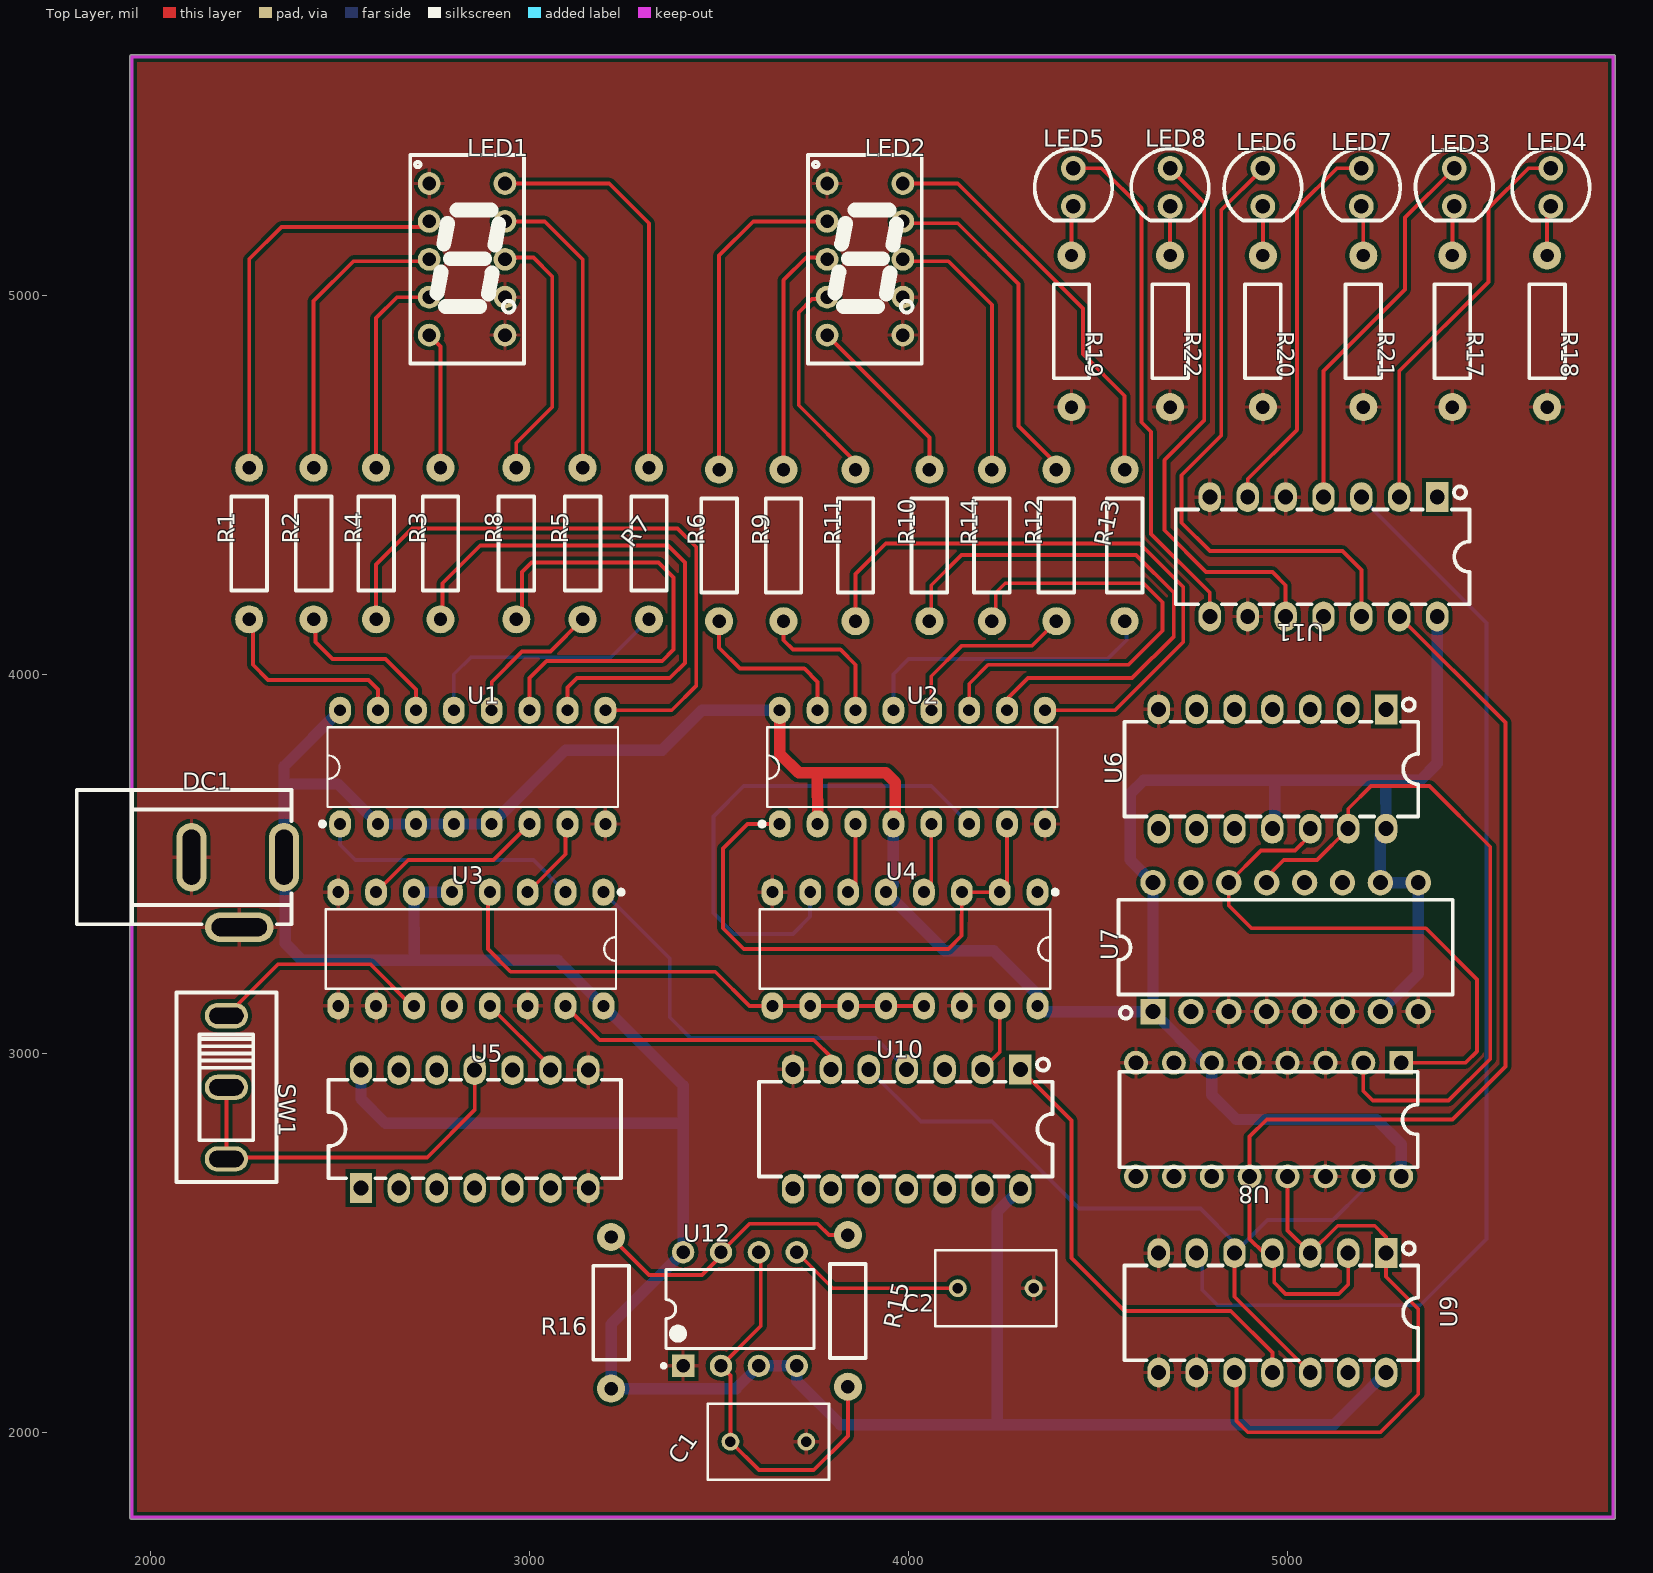
[diagram p0: Top Layer view]
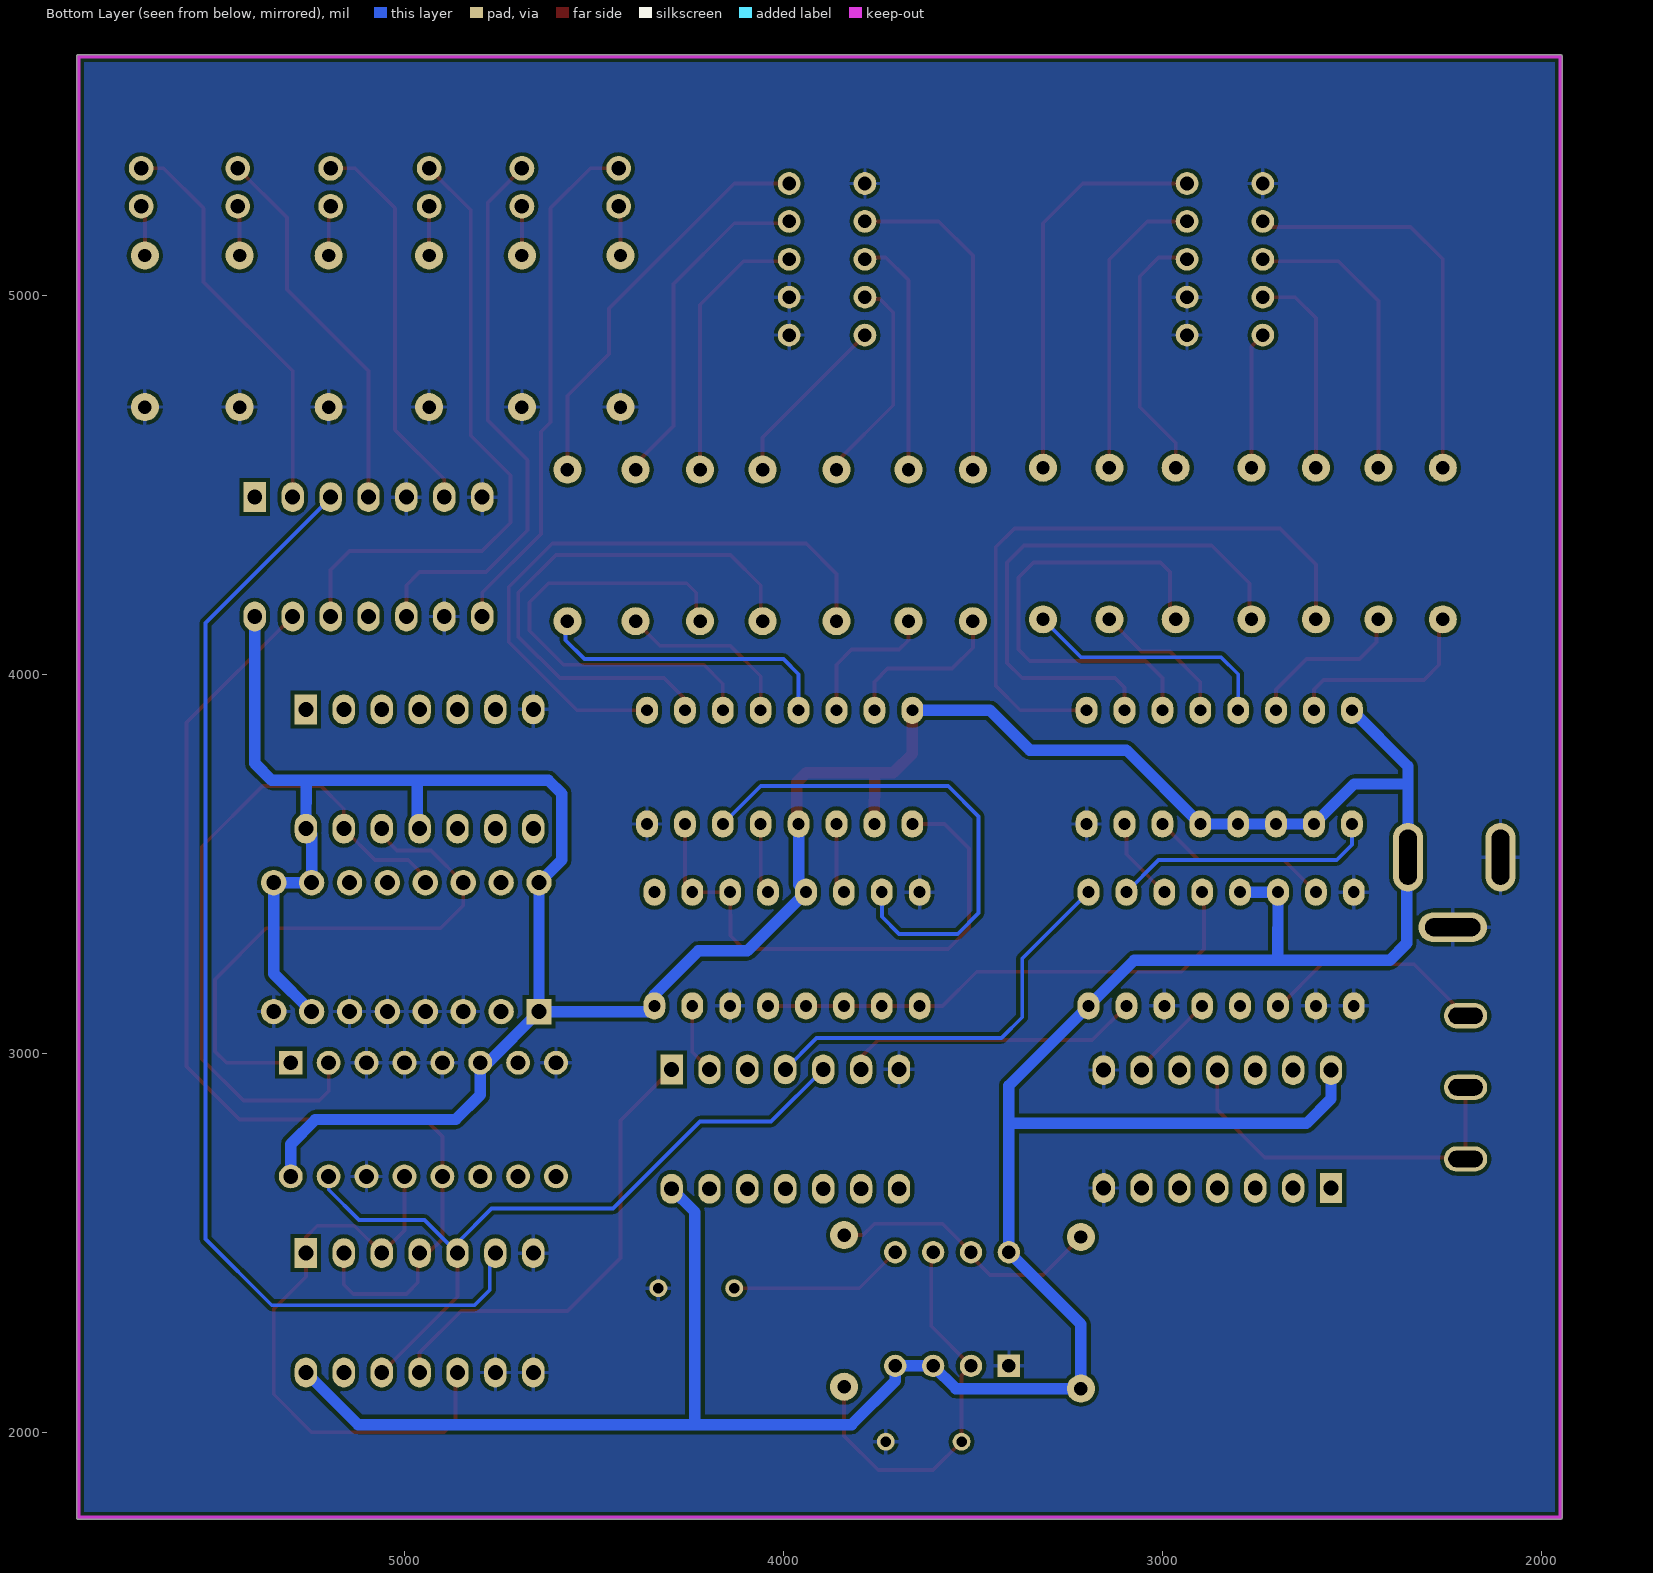
[diagram p1: Bottom Layer view, seen from below]
# Altium PCB MISC80800.pcbdoc
Units mil, origin at the board's own origin, x right, y up, seen from the top; angles counter-clockwise.
Board outline 3920.03 x 3865.03 mil, 2 copper layers (Top Layer, Bottom Layer); 46 components, 74 nets, 260 pads, 0 vias.

## Layer stack, top to bottom (the 12.6 mil dielectric is the usual default, probably not edited)
Top Solder: solder mask 0.4, Solder Resist, Dk 3.5
Top Layer: signal copper 1.4
Dielectric1: dielectric 12.6, FR-4, Dk 4.8
Bottom Layer: signal copper 1.4
Bottom Solder: solder mask 0.4, Solder Resist, Dk 3.5

## Board outline
1944.98,1775 ccw(c1950,1775) 1950,1769.98 5860,1769.98 ccw(c5860,1775) 5865.02,1775 5865.02,5630 ccw(c5860,5630) 5860,5635.02 1950,5635.02 ccw(c1950,5630) 1944.98,5630

## Design rules (kind name [scope] priority, off if disabled: settings)
Clearance [All] p1: gap=10
HoleSize [All] p1: absolutevalues=TRUE maxlimit=6666 minlimit=1 maxpercent=80.000 minpercent=20.000
MinimumSolderMaskSliver [All] p1: minsoldermaskwidth=0
PolygonConnect [All] p1: connectstyle=Relief reliefconductorwidth=10 reliefentries=4 polygonreliefangle="90 Angle" airgapwidth=10
RoutingVias [All] p1: holewidth=28 width=50 viastyle="Through Hole" minholewidth=28 minwidth=50 maxholewidth=28 maxwidth=50
SilkToSilkClearance [All] p1: silktosilkclearance=0
SilkToSolderMaskClearance [IsPad] p1: minsilkscreentomaskgap=0 clearancetoexposedcopper=TRUE
SolderMaskExpansion [All] p1: expansion=4
Width [All] p1: maxlimit=50 minlimit=10 preferedwidth=10
26 further rules are at their usual default settings.

## Components (designator, comment, footprint, x,y, rotation, side; value= is the part's Value field where it differs from the comment)
C1 "10U" RAD-0.2 3630,1975 r180 top
C2 "10N" RAD-0.2 4230,2380 r180 top
DC1 "DC005-2.0MM" DC-IN-TH_DC005 2230,3425 r0 top
LED1 "FJ3161AH" LED-SEG-TH_10P-L14.0-W7.5-P2.54-S5.08-TL 2835,5095 r0 top
LED2 "FJ3161AH" LED-SEG-TH_10P-L14.0-W7.5-P2.54-S5.08-TL 3885,5095 r0 top
LED3 "LED-TH-5mm_R" LED-TH_BD5.0_RED 5440,5285 r0 top
LED4 "LED-TH-5mm_R" LED-TH_BD5.0_RED 5695,5284.99 r0 top
LED5 "LED-TH-5mm_R" LED-TH_BD5.0_RED 4435,5284.99 r0 top
LED6 "LED-TH-5mm_R" LED-TH_BD5.0_RED 4935,5284.99 r0 top
LED7 "LED-TH-5mm_R" LED-TH_BD5.0_RED 5195,5284.99 r0 top
LED8 "LED-TH-5mm_R" LED-TH_BD5.0_RED 4690,5285 r0 top
R1 "330" R_AXIAL-0.4 2260,4345 r90 top
R2 "330" R_AXIAL-0.4 2430,4345 r90 top
R3 "330" R_AXIAL-0.4 2765,4345 r90 top
R4 "330" R_AXIAL-0.4 2595,4345 r90 top
R5 "330" R_AXIAL-0.4 3140,4345 r90 top
R6 "330" R_AXIAL-0.4 3500,4340 r90 top
R7 "330" R_AXIAL-0.4 3315,4345 r90 top
R8 "330" R_AXIAL-0.4 2965,4345 r90 top
R9 "330" R_AXIAL-0.4 3670,4340 r90 top
R10 "330" R_AXIAL-0.4 4055,4340 r90 top
R11 "330" R_AXIAL-0.4 3860,4340 r90 top
R12 "330" R_AXIAL-0.4 4390,4340 r90 top
R13 "330" R_AXIAL-0.4 4570,4340 r90 top
R14 "330" R_AXIAL-0.4 4220,4340 r90 top
R15 "50K" R_AXIAL-0.4 3840,2320 r270 top
R16 "50K" R_AXIAL-0.4 3215,2315 r90 top
R17 "200" R_AXIAL-0.4 5435,4905 r270 top
R18 "200" R_AXIAL-0.4 5685,4905 r270 top
R19 "200" R_AXIAL-0.4 4430,4905 r270 top
R20 "200" R_AXIAL-0.4 4935,4905 r270 top
R21 "200" R_AXIAL-0.4 5200,4905 r270 top
R22 "200" R_AXIAL-0.4 4690,4905 r270 top
SW1 "SS12D10G4 071" SW-TH_SHOU-HAN_SS12D10G4 2200,2910 r270 top
U1 "XD74LS48" DIP-16_L19.3-W6.4-P2.54-LS7.6-BL 2850,3755 r0 top
U2 "XD74LS48" DIP-16_L19.3-W6.4-P2.54-LS7.6-BL 4010,3755 r0 top
U3 "XD74LS192" DIP-16_L19.3-W6.4-P2.54-LS7.6-BL 2845,3275 r180 top
U4 "XD74LS192" DIP-16_L19.3-W6.4-P2.54-LS7.6-BL 3990.56,3275 r180 top
U5 "SN74LS32N" PDIP-14_L19.6-W6.5-P2.54-LS7.9-BL 2855,2800 r0 top
U6 "SN74LS00N" PDIP-14_L19.7-W6.6-P2.54-LS8.3-BL 4960,3750 r180 top
U7 "SN74LS160N(LX)" DIP-16_L22.4-W6.4-P2.54-LS8.64-BL 4995,3280 r0 top
U8 "XD74LS138" DIP-16_L19.8-W6.5-P2.54-LS7.6-BL 4950,2825 r180 top
U9 "SN74LS00N" PDIP-14_L19.7-W6.6-P2.54-LS8.3-BL 4960,2315 r180 top
U10 "SN74LS04N" PDIP-14_L19.7-W6.6-P2.54-LS8.3-BL 3995,2800 r180 top
U11 "SN74LS04N" PDIP-14_L19.7-W6.6-P2.54-LS8.3-BL 5095,4310 r180 top
U12 "100kHz" DIP-8_L9.8-W6.6-P2.54-LS7.6-BL 3555,2325 r0 top

## Footprints (in the part's own frame and the unit in brackets; to place one, negate y for a bottom-side part, rotate by r counter-clockwise, add the part's x,y. Pads: shape width x height; smd on the part's side, far side on the other; paste and mask are expansions set on the pad)
DC-IN-TH_DC005 [mm]
  oval 2x4.6 hole 1.2 slot 3.7 at 90 deg paste+0 mask+0.051: 1(3.1,2.35) 2(-3.1,2.35)
  oval 4.6x2 hole 1.2 slot 3.7 at 0 deg paste+0 mask+0.051: 3(0.1,-2.35)
  silkscreen extent -10.8,-2.15 3.6,6.85
DIP-8_L9.8-W6.6-P2.54-LS7.6-BL [mm]
  rect 1.5x1.5 hole 0.9 paste+0 mask+0.051: 1(-3.81,-3.81)
  round 1.5 hole 0.9 paste+0 mask+0.051: 2(-1.27,-3.81) 3(1.27,-3.81) 4(3.81,-3.81) 5(3.81,3.81) 6(1.27,3.81) 7(-1.27,3.81) 8(-3.81,3.81)
  silkscreen extent -5.23,-3.93 4.96,2.65
DIP-16_L19.3-W6.4-P2.54-LS7.6-BL [mm]
  oval 1.46x1.825 hole 0.8 paste+0 mask+0.051: 1(-8.89,-3.81) 2(-6.35,-3.81) 3(-3.81,-3.81) 4(-1.27,-3.81) 5(1.27,-3.81) 6(3.81,-3.81) 7(6.35,-3.81) 8(8.89,-3.81) 9(8.89,3.81) 10(6.35,3.81) 11(3.81,3.81) 12(1.27,3.81) 13(-1.27,3.81) 14(-3.81,3.81) 15(-6.35,3.81) 16(-8.89,3.81)
  silkscreen extent -10.22,-3.96 9.73,2.67
DIP-16_L19.8-W6.5-P2.54-LS7.6-BL [mm]
  rect 1.6x1.6 hole 1 paste+0 mask+0.051: 1(-8.89,-3.81)
  round 1.6 hole 1 paste+0 mask+0.051: 2(-6.35,-3.81) 3(-3.81,-3.81) 4(-1.27,-3.81) 5(1.27,-3.81) 6(3.81,-3.81) 7(6.35,-3.81) 8(8.89,-3.81) 9(8.89,3.81) 10(6.35,3.81) 11(3.81,3.81) 12(1.27,3.81) 13(-1.27,3.81) 14(-3.81,3.81) 15(-6.35,3.81) 16(-8.89,3.81)
  silkscreen extent -10,-3.2 10,3.2
DIP-16_L22.4-W6.4-P2.54-LS8.64-BL [mm]
  rect 1.7x1.7 hole 1 paste+0 mask+0.051: 1(-8.89,-4.32)
  round 1.7 hole 1 paste+0 mask+0.051: 2(-6.35,-4.32) 3(-3.81,-4.32) 4(-1.27,-4.32) 5(1.27,-4.32) 6(3.81,-4.32) 7(6.35,-4.32) 8(8.89,-4.32) 9(8.89,4.32) 10(6.35,4.32) 11(3.81,4.32) 12(1.27,4.32) 13(-1.27,4.32) 14(-3.81,4.32) 15(-6.35,4.32) 16(-8.89,4.32)
  silkscreen extent -11.21,-4.79 11.2,3.18
LED-SEG-TH_10P-L14.0-W7.5-P2.54-S5.08-TL [mil]
  round 60 hole 36 paste+0 mask+2: 1(-100,200) 2(-100,100) 3(-100,0) 4(-100,-100) 5(-100,-200) 6(100,-200) 7(100,-100) 8(100,0) 9(100,100) 10(100,200)
  silkscreen extent -150,-275 150,275
LED-TH_BD5.0_RED [mil]
  round 65 hole 38 paste+0 mask+2: 1(0,50) 2(0,-50)
  silkscreen extent -102,-88 102,102
PDIP-14_L19.6-W6.5-P2.54-LS7.9-BL [mm]
  rect 1.5x2 hole 1 paste+0 mask+0.051: 1(-7.62,-3.95)
  oval 1.5x2 hole 1 paste+0 mask+0.051: 2(-5.08,-3.95) 3(-2.54,-3.95) 4(0,-3.95) 5(2.54,-3.95) 6(5.08,-3.95) 7(7.62,-3.95) 8(7.62,3.95) 9(5.08,3.95) 10(2.54,3.95) 11(0,3.95) 12(-2.54,3.95) 13(-5.08,3.95) 14(-7.62,3.95)
  silkscreen extent -9.8,-3.3 9.8,3.3
PDIP-14_L19.7-W6.6-P2.54-LS8.3-BL [mm]
  rect 1.5x2 hole 1 paste+0 mask+0.051: 1(-7.62,-4)
  oval 1.5x2 hole 1 paste+0 mask+0.051: 2(-5.08,-4) 3(-2.54,-4) 4(0,-4) 5(2.54,-4) 6(5.08,-4) 7(7.62,-4) 8(7.62,4) 9(5.08,4) 10(2.54,4) 11(0,4) 12(-2.54,4) 13(-5.08,4) 14(-7.62,4)
  silkscreen extent -9.78,-4.72 9.91,3.18
R_AXIAL-0.4 [mil]
  round 74 hole 35.4 paste+0 mask+2: 1(-200,0) 2(200,0)
  silkscreen extent -124,-47 124,47
RAD-0.2 [mm]
  round 1.2 hole 0.7 paste+0 mask+0.05: 1(2.54,0) 2(-2.54,0)
  silkscreen extent -4.06,-2.54 4.06,2.54
SW-TH_SHOU-HAN_SS12D10G4 [mm]
  oval 1.7x2.9 hole 1.1 slot 2.3 at 90 deg paste+0 mask+0.05: 1(-4.8,0) 2(0,0) 3(4.8,0)
  silkscreen extent -6.35,-3.35 6.35,3.35

## Nets (pads, with @x,y where several pads share a name; then routed paths per layer and width w, separated by ;. In a path a pad name is that pad's centre, name@x,y a point inside that pad or via, vN(x,y) a via of type N, cw(c..) or ccw(c..) an arc to the next point about the centre after c; other vN are vias at no path point)
GND: C1.2 C2.2 DC1.2 DC1.3 LED1.1 LED1.6 LED1.7 LED2.1 LED2.6 LED2.7 R17.2 R18.2 R19.2 R20.2 R21.2 R22.2 U1.8 U2.8 U3.8 U3.9 U3.10 U3.14 U4.8 U4.14 U5.7 U5.8 U6.7 U7.3 U7.4 U7.5 U7.6 U7.8 U8.3 U8.4 U8.5 U8.8 U8.14 U9.7 U9.8 U9.9 U10.7 U11.5 U11.7 U11.9 U12.1
LED1_2: LED1.2 R1.2 | length 1066.4
  Top Layer w10: R1.2 2260,5095 2345,5180 2720,5180 LED1.2
LED1_3: LED1.3 R2.2 | length 790.6
  Top Layer w10: R2.2 2430,4985 2535,5090 2730,5090 LED1.3
LED1_4: LED1.4 R4.2 | length 557.8
  Top Layer w10: R4.2 2595,4940 2650,4995 LED1.4
LED1_5: LED1.5 R3.2 | length 362.4
  Top Layer w10: LED1.5 2765,4865 R3.2
LED1_8: LED1.8 R8.2 | length 692.1
  Top Layer w10: LED1.8 2940,5100 3010,5100 3060,5050 3060,4705 2965,4610 R8.2
LED1_9: LED1.9 R5.2 | length 796.4
  Top Layer w10: LED1.9 3040,5195 3140,5095 R5.2
LED1_10: LED1.10 R7.2 | length 1068.5
  Top Layer w10: LED1.10 3210,5295 3315,5190 R7.2
LED2_2: LED2.2 R6.2 | length 887.3
  Top Layer w10: R6.2 3500,5105 3590,5195 LED2.2
LED2_3: LED2.3 R9.2 | length 641.9
  Top Layer w10: R9.2 3670,5040 3730,5100 3780,5100 LED2.3
LED2_4: LED2.4 R11.2 | length 568.7
  Top Layer w10: LED2.4 3780,4990 3745,4990 3710,4955 3710,4710 3860,4560 R11.2
LED2_5: LED2.5 R10.2 | length 466.8
  Top Layer w10: LED2.5 4055,4625 R10.2
LED2_8: LED2.8 R14.2 | length 719.7
  Top Layer w10: LED2.8 3990,5090 4105,5090 4220,4975 R14.2
LED2_9: LED2.9 R12.2 | length 904.8
  Top Layer w10: LED2.9 3990,5190 4130,5190 4290,5030 4290,4655 4390,4555 R12.2
LED2_10: LED2.10 R13.2 | length 1082.3
  Top Layer w10: LED2.10 4130,5295 4460,4965 4460,4845 4570,4735 R13.2
LED3_2: LED3.2 R17.1 | length 132.1
  Top Layer w10: R17.1 5435,5230 LED3.2
LED5_2: LED5.2 R19.1 | length 132.1
  Top Layer w10: R19.1 4430,5229.99 LED5.2
LED7_2: LED7.2 R21.1 | length 132.1
  Top Layer w10: LED7.2 5200,5229.99 R21.1
R1_1: R1.1 U1.15 | length 536.1
  Top Layer w10: R1.1 2270,4135 2270,4025 2310,3985 2575,3985 2600,3960 U1.15
R2_1: R2.1 U1.14 | length 433.8
  Top Layer w10: R2.1 2435,4140 2435,4085 2480,4040 2620,4040 2700,3960 U1.14
R3_1: R3.1 U1.10 | length 1459.1
  Top Layer w10: R3.1 2770,4150 2770,4240 2870,4340 3365,4340 3410,4295 3410,4030 3370,3990 3125,3990 3100,3965 U1.10
R4_1: R4.1 U1.9 | length 1682
  Top Layer w10: R4.1 2595,4290 2690,4385 3390,4385 3440,4335 3440,3970 3375,3905 U1.9
R5_1: R5.1 U1.12 | length 383.3
  Top Layer w10: U1.12 2900,3980 2980,4060 3055,4060 R5.1
R6_1: R6.1 U2.15 | length 442.3
  Top Layer w10: R6.1 3500,4070 3555,4015 3725,4015 3760,3980 U2.15
R7_1: R7.1 U1.13 | length 670.1
  Bottom Layer w10: U1.13 2800,4000 2845,4045 3215,4045 R7.1
R8_1: R8.1 U1.11 | length 1244.2
  Top Layer w10: R8.1 2980,4160 2980,4270 3005,4295 3340,4295 3380,4255 3380,4065 3350,4035 3045,4035 3000,3990 U1.11
R9_1: R9.1 U2.14 | length 386.9
  Top Layer w10: R9.1 3670,4090 3695,4065 3820,4065 3860,4025 U2.14
R10_1: R10.1 U2.10 | length 1465
  Top Layer w10: R10.1 4060,4145 4060,4235 4140,4315 4600,4315 4700,4215 4700,4100 4590,3990 4315,3990 4260,3935 U2.10
R11_1: R11.1 U2.9 | length 1655.3
  Top Layer w10: R11.1 3860,4265 3940,4345 4610,4345 4725,4230 4725,4085 4545,3905 U2.9
R12_1: R12.1 U2.12 | length 480.1
  Top Layer w10: U2.12 4060,3995 4140,4075 4325,4075 R12.1
R13_1: R13.1 U2.13 | length 799.4
  Bottom Layer w10: U2.13 3960,4000 4000,4040 4525,4040 4575,4090 4575,4135 R13.1
R14_1: R14.1 U2.11 | length 1263.2
  Top Layer w10: U2.11 4160,3975 4210,4025 4580,4025 4670,4115 4670,4190 4620,4240 4255,4240 4230,4215 4230,4150 R14.1
R18_1: LED4.2 R18.1 | length 134.1
  Top Layer w10: R18.1 5685,5224.99 LED4.2
R20_1: LED6.2 R20.1 | length 130
  Top Layer w10: R20.1 LED6.2
R22_1: LED8.2 R22.1 | length 130
  Top Layer w10: R22.1 LED8.2
S$8163: 
S$8170: 
S$8174: 
U1_1: U1.1 U3.2 | length 701.8
  Bottom Layer w10: U1.1 2500,3550 2540,3510 3010,3510 U3.2
U1_6: U1.6 U3.7 | length 479.6
  Top Layer w10: U3.7 2680,3510 2905,3510 U1.6
U1_7: U1.7 U3.3 | length 233.5
  Top Layer w10: U3.3 3095,3525 3095,3610 U1.7
U2_3: U2.3 U4.6 | length 188.1
  Top Layer w10: U4.6 3860,3444.44 U2.3
U2_5: U2.5 U4.4 | length 188.1
  Top Layer w10: U4.4 4060,3444.44 U2.5
U2_6: U2.6 U4.7 | length 1366
  Bottom Layer w10: U4.7 3740,3360 3695,3315 3540,3315 3485,3370 3485,3625 3565,3705 4060,3705 U2.6
U2_7: U2.1 U2.7 U4.2 U4.3 | length 1457.3
  Top Layer w10: U2.1 3575,3605 3510,3540 3510,3330 3565,3275 4105,3275 4140,3310 U4.3 ; U4.3 U4.2 4260,3444.44 U2.7
U3_1: U3.1 U10.4 | length 1084.5
  Bottom Layer w10: U3.1 3370,3250 3370,3095 3425,3040 3912.48,3040 U10.4
U3_4: U3.4 U4.9 U4.10 U4.11 U4.12 U4.13 | length 1364.8
  Top Layer w10: U3.4 2890,3420 2890,3275 2950,3215 3490,3215 3580,3125 U4.9 U4.13
U3_11: SW1.1 U3.11 | length 596.9
  Top Layer w10: SW1.1 2336.03,3235 2580,3235 2690,3125 U3.11
U3_13: U3.13 U5.9 | length 235.8
  Top Layer w10: U3.13 3055,2965 U5.9
U3_15: U3.15 U10.6 | length 788.4
  Top Layer w10: U3.15 3185,3035 3750,3035 3795,2990 U10.6
U4_1: U4.1
U4_15: U4.15 U10.2 | length 186.4
  Top Layer w10: U10.2 4240.56,3003.04 U4.15
U5_11: SW1.2 SW1.3 U5.11 | length 1002.9
  Top Layer w10: SW1.2 SW1.3 2203.97,2725 2730,2725 2855,2850 U5.11
U6_12: U6.12 U7.14 U8.1 | length 1482.6
  Top Layer w10: U6.12 5060,3575 5020,3535 4929.92,3535 U7.14 4845,3390 4905,3330 5365,3330 5500,3195 5500,3005 5470,2975 U8.1
U6_13: U6.13 U7.13 U8.2 | length 1827.3
  Top Layer w10: U7.13 4945,3465 4990,3510 5077.48,3510 U6.13 5160,3645 5220,3705 5375,3705 5535,3545 5535,2985 5425,2875 5225,2875 5200,2900 U8.2
U8_12: U8.12 U9.2 U9.4 U11.13 | length 2780.5
  Top Layer w10: U9.2 5160,2390 5135,2365 4995,2365 4965,2395 4965,2467.48 U9.4 4937.5,2472.5 4900,2510 4900,2780 4945,2825 5435,2825 5575,2965 5575,3872.5 U11.13
U8_13: U8.13 U9.1 U9.3 U9.10 | length 1583.5
  Top Layer w10: U9.10 4865,2152.52 4865,2030 4895,2000 5245,2000 5345,2100 5345,2325 5260,2410 U9.1 5260,2515 5230,2545 5132.52,2545 U9.3 5000,2532.48 U8.13
U8_15: U8.15 U9.5 U9.12 U10.5 | length 2024.2
  Top Layer w10: U9.5 4860,2357.52 U9.12
  Bottom Layer w10: U10.5 4032.48,2820 4220,2820 4450,2590 4770,2590 4860,2500 U9.5 4947.52,2560 5120,2560 5200,2640 U8.15
U9_6: U9.6 U11.3 | length 3037
  Bottom Layer w10: U9.6 4775,2457.5 4775,2375 4815,2335 5350,2335 5525,2510 5525,4135 5195,4465 U11.3
U9_11: U9.11 U10.1 | length 1239.4
  Top Layer w10: U10.1 4430,2822.48 4430,2460 4570,2320 4850,2320 4960,2210 U9.11
U9_13: U9.13
U10_3: U10.3
U11_1: U11.1
U11_2: LED4.1 U11.2 | length 1068.3
  Top Layer w10: U11.2 5295,4800 5530,5035 5530,5230 5635,5335 LED4.1
U11_4: LED3.1 U11.4 | length 1010.4
  Top Layer w10: U11.4 5095,4800 5310,5015 5310,5205 LED3.1
U11_6: LED7.1 U11.6 | length 1029.8
  Top Layer w10: U11.6 4895,4515 5025,4645 5025,5230 5130,5335 LED7.1
U11_8: LED5.1 U11.8 | length 1375.6
  Top Layer w10: LED5.1 4510,5335 4615,5230 4615,4665 4640,4640 4640,4370 4795,4215 U11.8
U11_10: LED8.1 U11.10 | length 1498.3
  Top Layer w10: LED8.1 4780,5245 4780,4670 4675,4565 4675,4380 4785,4270 4960,4270 4995,4235 U11.10
U11_11: U11.11
U11_12: LED6.1 U11.12 | length 1673.3
  Top Layer w10: LED6.1 4825,5224.99 4825,4630 4720,4525 4720,4400 4795,4325 5145,4325 5195,4275 U11.12
U12_2: C1.1 R15.2 U12.2 U12.6 | length 1074.3
  Top Layer w10: U12.6 3610,2480 3610,2280 U12.2 3530,2150 C1.1 3605,1900 3750,1900 3840,1990 R15.2
U12_5: C2.1 U12.5 | length 464.4
  Top Layer w10: U12.5 3800,2380 C2.1
U12_7: R15.1 R16.2 U12.7 | length 740.6
  Top Layer w10: R16.2 3315,2415 3455,2415 3505,2465 U12.7 3580,2550 3760,2550 3790,2520 R15.1
VCC: DC1.1 R16.1 U1.2 U1.3 U1.4 U1.5 U1.16 U2.2 U2.4 U2.16 U3.5 U3.6 U3.16 U4.5 U4.16 U5.14 U6.11 U6.14 U7.1 U7.7 U7.9 U7.10 U7.16 U8.6 U8.16 U9.14 U10.14 U11.14 U12.3 U12.4 U12.8 | length 13725
  Top Layer w30: U2.16 3660,3790 3710,3740 3940,3740 3965,3715 3965,3610 U2.4 ; 3759.5,3740 U2.2
  Bottom Layer w30: 2352.04,3710.62 2494.38,3710.62 U1.2 U1.4 U1.5 3095,3800 3350,3800 3455,3905 U2.16 ; U1.16 2352.04,3757.04 DC1.1 2355,3514.55 2355,3290 2400,3245 3075,3245 U3.16 3405,2915 U12.8 3215,2285 R16.1 3545,2115 U12.3 U12.4 3705,2135 3820,2020 5122.48,2020 U9.14 ; U5.14 2555,2880 2620,2815 3402.2,2815 3405,2812.2 ; 2695.2,3245 U3.6 U3.5 ; U2.4 3960,3444.44 U4.5 4095.56,3270 4225,3270 4340.56,3154.44 U4.16 4355.64,3109.92 U7.1 ; 4233.62,2020 4233.62,2581.14 U10.14 ; U6.11 4966.13,3598.65 4966.13,3720 ; U7.7 5345,3209.92 U7.9 U7.10 5245,3577.52 U6.14 5259.5,3720 ; U8.16 5300,2760 5235,2825 4865,2825 4800,2890 U8.6 4779.92,2975 U7.1 ; U11.14 5395,3765 5350,3720 4620,3720 4585,3685 4585,3510.08 U7.16 U7.1
pads on no net: U3.12 U5.1 U5.2 U5.3 U5.4 U5.5 U5.6 U5.10 U5.12 U5.13 U6.1 U6.2 U6.3 U6.4 U6.5 U6.6 U6.8 U6.9 U6.10 U7.2 U7.11 U7.12 U7.15 U8.7 U8.9 U8.10 U8.11 U10.8 U10.9 U10.10 U10.11 U10.12 U10.13

## Polygon pours and split planes (outlines as drawn)
GND on Bottom Layer "D" (solid, remove dead copper, pour order 4): 1630,5785 1705,5860 6270,5860 6270,1870 6130,1730 6065,1665 1520,1665
GND on Top Layer "D" (solid, remove dead copper, pour order 6): 1470,5860 5730,5860 5775,5815 5790,5830 5970,5830 5970,1565 6075,1460 5975,1360 1555,1360